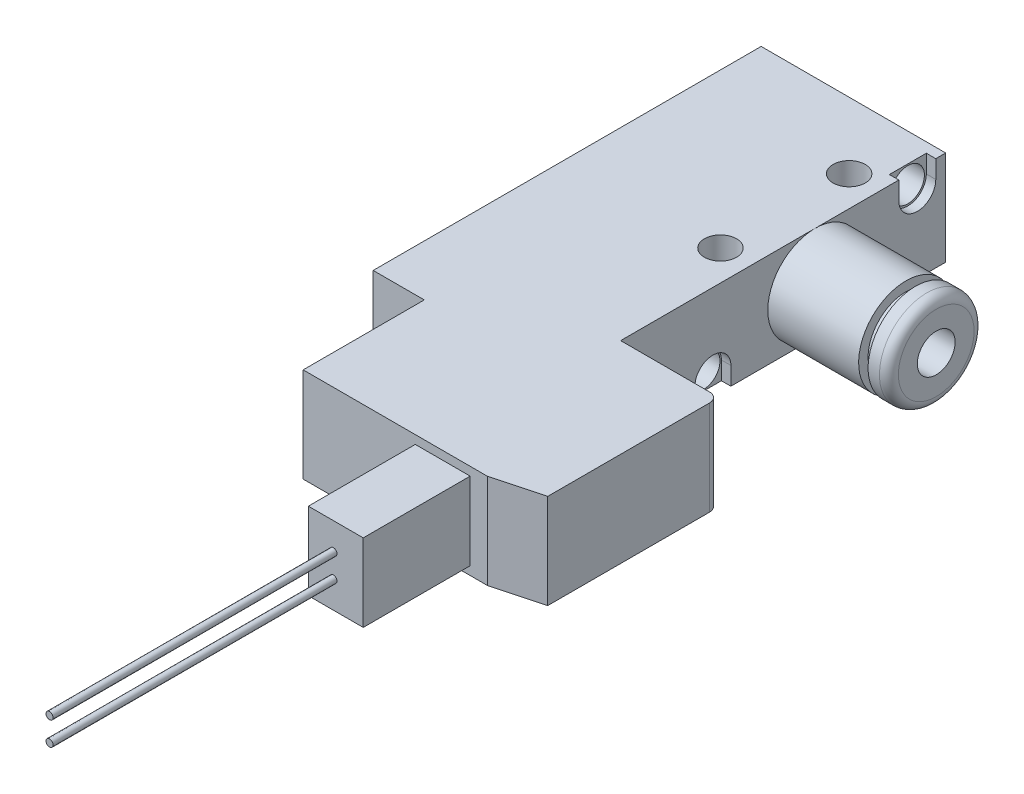
from build123d import *

# Parameters (mm, degrees)
SKETCH1_W             = 53.8
SKETCH1_H             = 10
BOSS_EXTRUDE1_DEPTH   = 29.9
SKETCH2_R             = 1.7
CUT_EXTRUDE1_DEPTH    = 29.9
SKETCH5_W             = 5.4
SKETCH5_H             = 12.8
CUT_EXTRUDE3_DEPTH    = 30
M5_TAPPED_HOLE1_D     = 4.2
M5_TAPPED_HOLE1_DEPTH = 12.4
M5_TAPPED_HOLE1_TIP   = 1.2618073
SKETCH3_W             = 5.8
SKETCH3_H             = 8.2
BOSS_EXTRUDE4_DEPTH   = 11.3
SKETCH7_R             = 0.375
BOSS_EXTRUDE5_DEPTH   = 30
SKETCH8_W             = 10.4
SKETCH8_H             = 34.35
CUT_EXTRUDE4_DEPTH    = 30
SKETCH9_R             = 5
SKETCH9_R_2           = 2
BOSS_EXTRUDE6_DEPTH   = 12.8
FILLET1_R             = 1
FILLET2_R             = 1
CHAMFER2_SIZE         = 5
CHAMFER2_SIZE2        = 1.339745962
SKETCH11_W            = 1
SKETCH11_H            = 1
SKETCH12_R            = 1.75
CUT_EXTRUDE5_DEPTH    = 10
CUT_EXTRUDE6_DEPTH    = 1


with BuildPart() as part:
    # Sketch1 → Boss-Extrude1 (new body)
    with BuildSketch(Plane(origin=(0, 0, 0), x_dir=(0, 0, -1), z_dir=(1, 0, 0))):
        Rectangle(SKETCH1_W, SKETCH1_H)
    extrude(amount=BOSS_EXTRUDE1_DEPTH)

    # Sketch2 → Cut-Extrude1 (cut)
    with BuildSketch(Plane.XZ.offset(5)):
        with Locations(Location((16.3, -19.9, 0), (0, 0, 270))):
            Circle(SKETCH2_R)
        with Locations(Location((16.3, -6.3, 0), (0, 0, 270))):
            Circle(SKETCH2_R)
    extrude(amount=-CUT_EXTRUDE1_DEPTH, mode=Mode.SUBTRACT)

    # Sketch5 → Cut-Extrude3 (cut)
    with BuildSketch(Plane.XZ.offset(5)):
        with Locations((2.7, 20.5)):
            Rectangle(SKETCH5_W, SKETCH5_H)
    extrude(amount=-CUT_EXTRUDE3_DEPTH, mode=Mode.SUBTRACT)

    # M5 Tapped Hole1
    with Locations(Plane(origin=(0, 0, -17.9), x_dir=(0, 0, -1), z_dir=(-1, 0, 0))):
        with Locations((0, 0), (-10.7, 0), (-23, 0)):
            Hole(M5_TAPPED_HOLE1_D / 2, depth=M5_TAPPED_HOLE1_DEPTH)
            with Locations((0, 0, -(M5_TAPPED_HOLE1_DEPTH + M5_TAPPED_HOLE1_TIP / 2))):  # 118° drill point
                Cone(0, M5_TAPPED_HOLE1_D / 2, M5_TAPPED_HOLE1_TIP, mode=Mode.SUBTRACT)

    # Sketch3 → Boss-Extrude4 (add)
    with BuildSketch(Plane.XY.offset(26.9)):
        with Locations((20.15, 0)):
            Rectangle(SKETCH3_W, SKETCH3_H)
    extrude(amount=BOSS_EXTRUDE4_DEPTH)

    # Sketch7 → Boss-Extrude5 (add)
    with BuildSketch(Plane.XY.offset(38.2)):
        with Locations((19.9, 1.25)):
            Circle(SKETCH7_R)
        with Locations((19.9, -1.25)):
            Circle(SKETCH7_R)
    extrude(amount=BOSS_EXTRUDE5_DEPTH)

    # Sketch8 → Cut-Extrude4 (cut)
    with BuildSketch(Plane.XZ.offset(5)):
        with Locations((24.7, -9.725)):
            Rectangle(SKETCH8_W, SKETCH8_H)
    extrude(amount=-CUT_EXTRUDE4_DEPTH, mode=Mode.SUBTRACT)

    # Sketch9 → Boss-Extrude6 (add)
    with BuildSketch(Plane(origin=(19.5, 0, 0), x_dir=(0, 0, -1), z_dir=(1, 0, 0))):
        with Locations(Location((13.1, 0, 0), (0, 0, 270))):
            Circle(SKETCH9_R)
        with Locations((13.1, 0)):
            Circle(SKETCH9_R_2, mode=Mode.SUBTRACT)
    extrude(amount=BOSS_EXTRUDE6_DEPTH)

    # Fillet1
    fillet1_edges = [part.edges().sort_by_distance(p)[0] for p in [
        (32.3, 5, -13.1),
    ]]
    fillet(fillet1_edges, radius=FILLET1_R)

    # Fillet2
    fillet2_edges = [part.edges().sort_by_distance(p)[0] for p in [
        (29.9, 0, 7.45),
    ]]
    fillet(fillet2_edges, radius=FILLET2_R)

    # Chamfer2
    chamfer2_edges = [part.edges().sort_by_distance(p)[0] for p in [
        (29.9, 0, 26.9),
    ]]
    chamfer2_side = [part.faces().sort_by_distance(p)[0] for p in [
        (17.047791734, 0, 26.9),
    ]]
    chamfer(chamfer2_edges, length=CHAMFER2_SIZE, length2=CHAMFER2_SIZE2, reference=chamfer2_side[0])

    # Sketch11 → Cut-Revolve1 (revolve, cut)
    with BuildSketch(Plane(origin=(0, 0, 0), x_dir=(1, 0, 0), z_dir=(0, 1, 0)), mode=Mode.PRIVATE) as cut_revolve1_sk:
        with Locations((29.6, 8.6)):
            Rectangle(SKETCH11_W, SKETCH11_H)
    revolve(cut_revolve1_sk.sketch.rotate(Axis((32.3, 0, -13.1), (-1, 0, 0)), 180), axis=Axis((32.3, 0, -13.1), (-1, 0, 0)), mode=Mode.SUBTRACT)

    # Sketch12 → Cut-Extrude5 (cut)
    with BuildSketch(Plane(origin=(19.5, 0, 0), x_dir=(0, 0, -1), z_dir=(1, 0, 0))):
        with Locations((23.9, 3.1)):
            Circle(SKETCH12_R)
        with Locations((2.3, -3.1)):
            Circle(SKETCH12_R)
    extrude(amount=-CUT_EXTRUDE5_DEPTH, mode=Mode.SUBTRACT)

    # Sketch13 → Cut-Extrude6 (cut)
    with BuildSketch(Plane(origin=(19.5, 0, 0), x_dir=(0, 0, -1), z_dir=(1, 0, 0))):
        with BuildLine():
            Line((4.2, -3.1), (4.2, -5))
            Line((4.2, -5), (0.4, -5))
            Line((0.4, -5), (0.4, -3.1))
            ThreePointArc((0.4, -3.1), (2.3, -1.2), (4.2, -3.1))
        make_face()
        with BuildLine():
            Line((25.852743459, 3.1), (25.852743459, 5))
            Line((25.852743459, 5), (21.947256541, 5))
            Line((21.947256541, 5), (21.947256541, 3.1))
            ThreePointArc((21.947256541, 3.1), (23.9, 1.147256541), (25.852743459, 3.1))
        make_face()
    extrude(amount=-CUT_EXTRUDE6_DEPTH, mode=Mode.SUBTRACT)


solid = part.part
